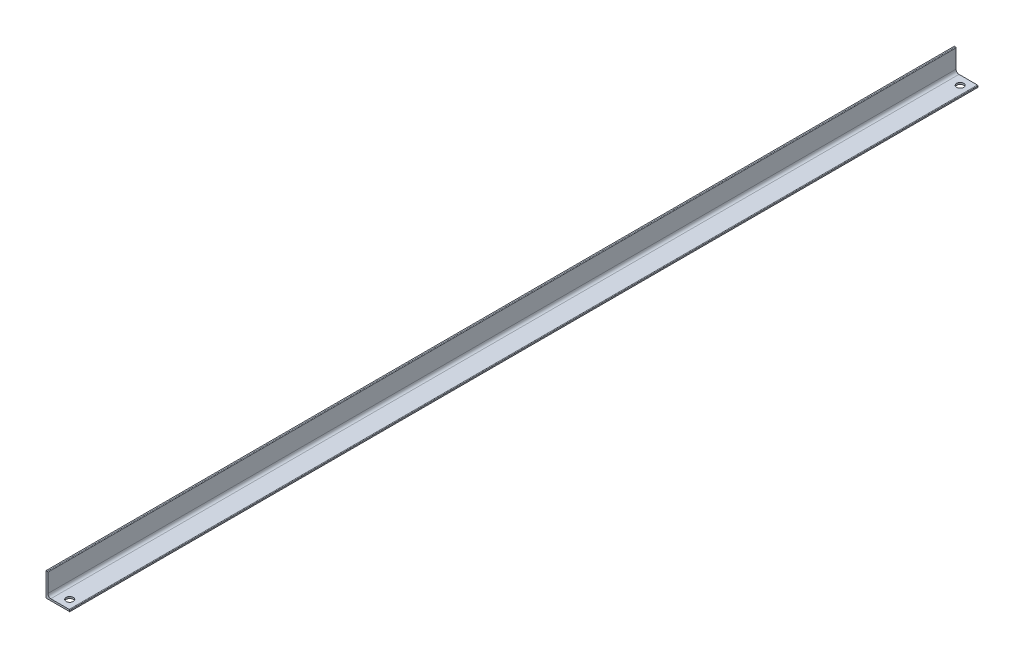
from build123d import *

# Parameters (mm, degrees)
BOSS_EXTRUDE1_DEPTH = 1530
SKETCH_1_R          = 6
CUT_EXTRUDE1_DEPTH  = 1532.045394494


with BuildPart() as part:
    # Sketch1 → Boss-Extrude1 (new body)
    with BuildSketch(Plane.XY):
        with BuildLine():
            Line((0, 0), (0, 40))
            Line((0, 40), (2, 40))
            ThreePointArc((2, 40), (2.707106781, 39.707106781), (3, 39))
            Line((3, 39), (3, 8))
            ThreePointArc((3, 8), (4.464466094, 4.464466094), (8, 3))
            Line((8, 3), (39, 3))
            ThreePointArc((39, 3), (39.707106781, 2.707106781), (40, 2))
            Line((40, 2), (40, 0))
            Line((40, 0), (0, 0))
        make_face()
    extrude(amount=BOSS_EXTRUDE1_DEPTH)

    # 草图1 → Cut-Extrude1 (cut, through all)
    with BuildSketch(Plane.XZ):
        with Locations(Location((25, 1515, 0), (0, 0, 270))):
            Circle(SKETCH_1_R)
        with Locations(Location((25, 15, 0), (0, 0, 270))):
            Circle(SKETCH_1_R)
    extrude(amount=-CUT_EXTRUDE1_DEPTH, mode=Mode.SUBTRACT)


solid = part.part
